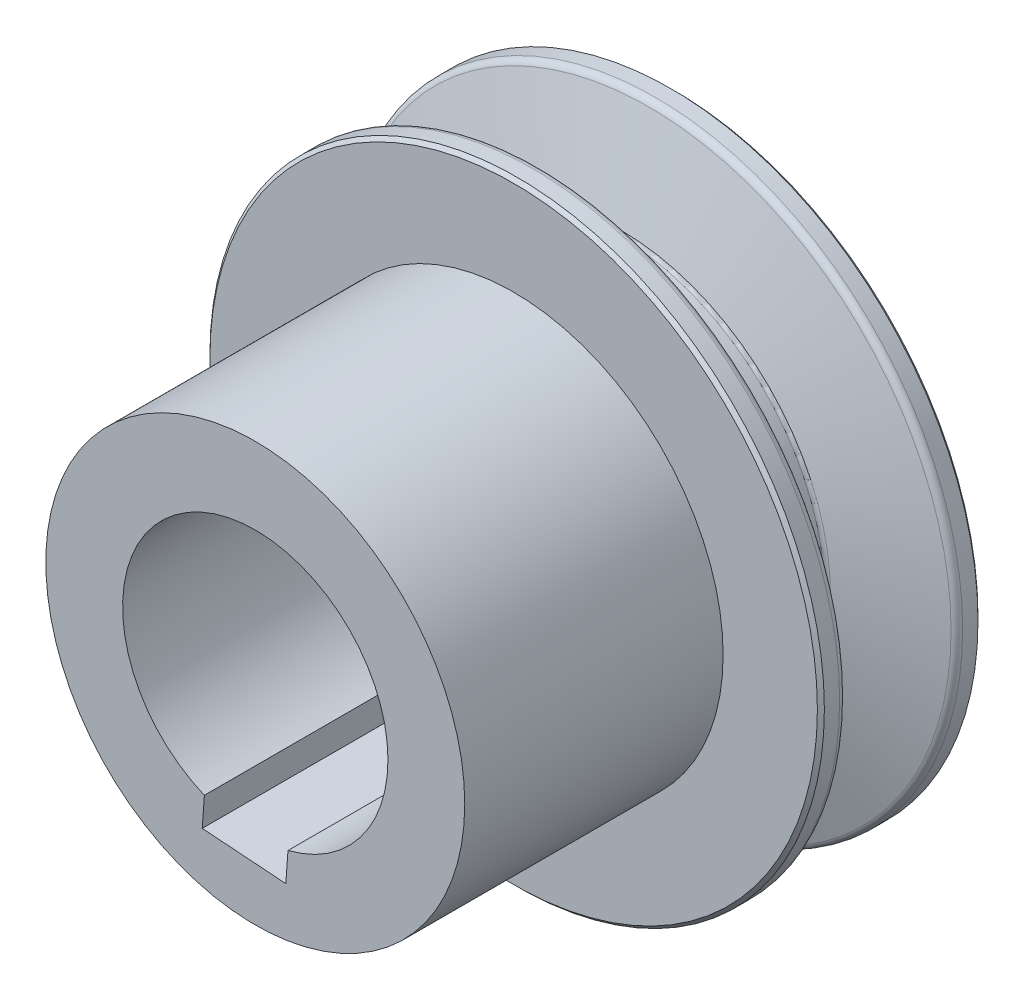
SolidWorks part; units mm, degrees
ref_plane "Front Plane" through (0, 0, 0) normal (0, 0, 1) x (1, 0, 0)
ref_plane "Top Plane" through (0, 0, 0) normal (0, 1, 0) x (1, 0, 0)
ref_plane "Right Plane" through (0, 0, 0) normal (1, 0, 0) x (0, 0, -1)
ref_plane "Plane1" through (0, 22.744, 0) normal (0, 1, 0) x (1, 0, 0)
sketch "Sketch1" plane through (0, 22.744, 0) normal (0, 1, 0) x (1, 0, 0)
  line L0 (620.2306, 121.693) -> (576.2306, 121.693)
  line L1 (576.2306, 121.693) -> (576.2306, 98.693)
  line L2 (576.2306, 98.693) -> (620.2306, 98.693)
  line L3 (620.2306, 98.693) -> (620.2306, 102.1229)
  line L4 (620.2306, 102.1229) -> (605.9306, 106.4949)
  line L5 (605.9306, 106.4949) -> (605.9306, 113.8911)
  line L6 (605.9306, 113.8911) -> (620.2306, 118.263)
  line L7 (620.2306, 118.263) -> (620.2306, 121.693)
  line L8 (576.2306, 121.693) -> (576.2306, 98.693) construction
  dimension "D1" = 29.7
  dimension "D2" = 44
  dimension "D3" = 3.4299
  dimension "D4" = 7.8019
  dimension "D5" = 15.1981
  dimension "D6" = 19.5701
  dimension "D7" = 23
revolve "Revolve1" add sketch "Sketch1" angle 360 about L8
sketch "Sketch2" plane through (0, 0, -98.693) normal (0, 0, 1) x (1, 0, 0)
  circle A0 centre (576.2306, 22.744) radius 30
  dimension "D1" = 60
extrude "Boss-Extrude1" add sketch "Sketch2" along normal blind 37
sketch "Sketch3" plane through (0, 0, -121.693) normal (0, 0, -1) x (-1, 0, 0)
  line L0 (-580.6029, 0.0686) -> (-568.6343, 0.9361)
  line L1 (-568.6343, 0.9361) -> (-568.9431, 5.1971)
  line L2 (-580.9117, 4.3296) -> (-580.6029, 0.0686)
  arc A0 (-568.9431, 5.1971) -> (-580.9117, 4.3296) centre (-576.2306, 22.744) cw
  circle A1 centre (-576.2306, 22.744) radius 44 construction
  dimension "D1" = 19
  dimension "D2" = 7.2875
  dimension "D3" = 7.5964
  dimension "D4" = 4.3722
  dimension "D5" = 4.6811
  dimension "D6" = 17.5468
  dimension "D7" = 18.4143
  dimension "D8" = 21.8079
  dimension "D9" = 22.6754
extrude "Cut-Extrude1" cut sketch "Sketch3" against normal through all
ref_plane "Plane2" through (0, 22.744, 0) normal (0, -1, 0) x (1, 0, 0)
sketch "Sketch4" plane through (0, 22.744, 0) normal (0, -1, 0) x (1, 0, 0)
  line L0 (595.2306, -61.693) -> (576.2306, -61.693)
  line L1 (576.2306, -61.693) -> (576.2306, -121.693)
  line L2 (576.2306, -121.693) -> (595.2306, -121.693)
  line L3 (595.2306, -121.693) -> (595.2306, -61.693)
  line L4 (576.2306, -61.693) -> (576.2306, -121.693) construction
  dimension "D1" = 19
  dimension "D2" = 60
revolve "Cut-Revolve1" cut sketch "Sketch4" angle 360 about L4
chamfer "Chamfer1" distance 0.5 angle 45 2 edges at (620.2306, 22.744, -98.693) (620.2306, 22.744, -121.693)
fillet "Fillet1" radius 0.5 2 edges at (605.9306, 22.744, -106.4949) (605.9306, 22.744, -113.8911)
fillet "Fillet2" radius 1 2 edges at (620.2306, 22.744, -102.1229) (620.2306, 22.744, -118.263)
sketch "Sketch5" plane through (0, 0, -61.693) normal (0, 0, 1) x (1, 0, 0)
  circle A0 centre (576.2306, 22.744) radius 30
